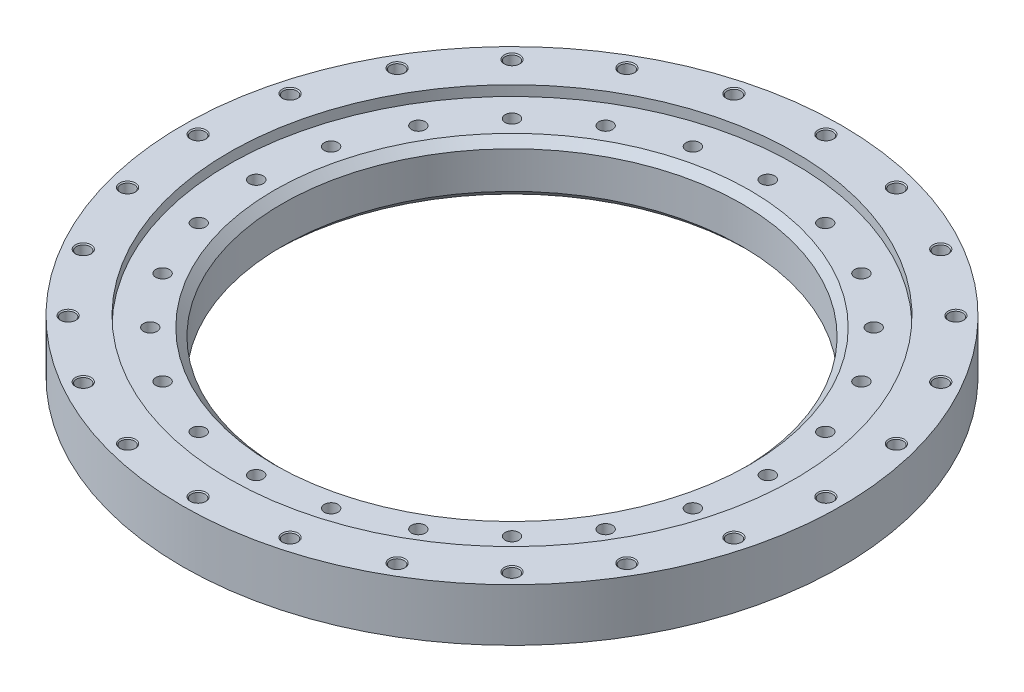
SolidWorks part; units mm, degrees
ref_plane "Front Plane" through (0, 0, 0) normal (0, 0, 1) x (1, 0, 0)
ref_plane "Top Plane" through (0, 0, 0) normal (0, 1, 0) x (1, 0, 0)
ref_plane "Right Plane" through (0, 0, 0) normal (1, 0, 0) x (0, 0, -1)
sketch "Sketch1" plane through (0, 0, 0) normal (0, 1, 0) x (1, 0, 0)
  circle A0 centre (0, 0) radius 420
  dimension "D1" = 840
extrude "Boss-Extrude1" add sketch "Sketch1" along normal blind 67
sketch "Sketch2" plane through (0, 67, 0) normal (0, 1, 0) x (1, 0, 0)
  circle A0 centre (0, 0) radius 360.5
  dimension "D1" = 721
extrude "Cut-Extrude1" cut sketch "Sketch2" against normal blind 13
sketch "Sketch3" plane through (0, 0, 0) normal (0, -1, 0) x (1, 0, 0)
  circle A0 centre (0, 0) radius 360
  dimension "D1" = 720
extrude "Boss-Extrude2" add sketch "Sketch3" along normal blind 13
hole_wizard "M20 Tapped Hole1" positions "Sketch4" profile "Sketch5" tap size "M20" standard "GB" end condition through all
sketch "Sketch4" plane through (0, 67, 0) normal (0, 1, 0) x (1, 0, 0)
  circle A0 centre (0, 0) radius 400 construction
  point P8 (0, 400)
  point P14 (103.5276, 386.3703)
  point P15 (200, 346.4102)
  point P16 (282.8427, 282.8427)
  point P17 (346.4102, 200)
  point P18 (386.3703, 103.5276)
  point P19 (400, 0)
  point P20 (386.3703, -103.5276)
  point P21 (346.4102, -200)
  point P22 (282.8427, -282.8427)
  point P23 (200, -346.4102)
  point P24 (103.5276, -386.3703)
  point P25 (0, -400)
  point P26 (-103.5276, -386.3703)
  point P27 (-200, -346.4102)
  point P28 (-282.8427, -282.8427)
  point P29 (-346.4102, -200)
  point P30 (-386.3703, -103.5276)
  point P31 (-400, 0)
  point P32 (-386.3703, 103.5276)
  point P33 (-346.4102, 200)
  point P34 (-282.8427, 282.8427)
  point P35 (-200, 346.4102)
  point P36 (-103.5276, 386.3703)
  dimension "D2" = 24
sketch "Sketch5" plane through (-103.5276, 67, -386.3703) normal (1, 0, 0) x (0, 0, 1)
  line L0 (0, 0) -> (0, 80)
  line L1 (0, 80) -> (8.75, 80)
  line L2 (8.75, 80) -> (8.75, 1.275)
  line L3 (8.75, 1.275) -> (10.025, 0)
  line L5 (10.025, 0) -> (0, 0)
  line L6 (-8.75, 1.275) -> (-10.025, 0) construction
  line L11 (0, -6.35) -> (0, 107.95) construction
  dimension "通孔螺纹孔钻头直径" = 17.5
  dimension "通孔螺纹孔钻头深度" = 80
  dimension "近端锥形沉头孔直径" = 20.05
  dimension "近端锥形沉头孔角度" = 90
cosmetic thread "Cosmetic thread 1" parameters "D2"=20
cosmetic thread "Cosmetic thread 2" parameters "D2"=20
cosmetic thread "Cosmetic thread 3" parameters "D2"=20
cosmetic thread "Cosmetic thread 4" parameters "D2"=20
cosmetic thread "Cosmetic thread 5" parameters "D2"=20
cosmetic thread "Cosmetic thread 6" parameters "D2"=20
cosmetic thread "Cosmetic thread 7" parameters "D2"=20
cosmetic thread "Cosmetic thread 8" parameters "D2"=20
cosmetic thread "Cosmetic thread 9" parameters "D2"=20
cosmetic thread "Cosmetic thread 10" parameters "D2"=20
cosmetic thread "Cosmetic thread 11" parameters "D2"=20
cosmetic thread "Cosmetic thread 12" parameters "D2"=20
cosmetic thread "Cosmetic thread 13" parameters "D2"=20
cosmetic thread "Cosmetic thread 14" parameters "D2"=20
cosmetic thread "Cosmetic thread 15" parameters "D2"=20
cosmetic thread "Cosmetic thread 16" parameters "D2"=20
cosmetic thread "Cosmetic thread 17" parameters "D2"=20
cosmetic thread "Cosmetic thread 18" parameters "D2"=20
cosmetic thread "Cosmetic thread 19" parameters "D2"=20
cosmetic thread "Cosmetic thread 20" parameters "D2"=20
cosmetic thread "Cosmetic thread 21" parameters "D2"=20
cosmetic thread "Cosmetic thread 22" parameters "D2"=20
cosmetic thread "Cosmetic thread 23" parameters "D2"=20
cosmetic thread "Cosmetic thread 24" parameters "D2"=20
sketch "Sketch6" plane through (0, 54, 0) normal (0, 1, 0) x (1, 0, 0)
  circle A0 centre (0, 0) radius 293
  dimension "D1" = 586
extrude "Cut-Extrude2" cut sketch "Sketch6" against normal through all
chamfer "Chamfer1" distance 10 angle 45 2 edges at (0, -13, 293) (0, 54, 293)
hole_wizard "M20 Tapped Hole2" positions "Sketch7" profile "Sketch8" tap size "M20" standard "GB" end condition through all
sketch "Sketch7" plane through (0, -13, 0) normal (0, -1, 0) x (-1, 0, 0)
  circle A0 centre (0, 0) radius 326 construction
  point P5 (0, 326)
  point P12 (84.375, 314.8918)
  point P13 (163, 282.3243)
  point P14 (230.5168, 230.5168)
  point P15 (282.3243, 163)
  point P16 (314.8918, 84.375)
  point P17 (326, 0)
  point P18 (314.8918, -84.375)
  point P19 (282.3243, -163)
  point P20 (230.5168, -230.5168)
  point P21 (163, -282.3243)
  point P22 (84.375, -314.8918)
  point P23 (0, -326)
  point P24 (-84.375, -314.8918)
  point P25 (-163, -282.3243)
  point P26 (-230.5168, -230.5168)
  point P27 (-282.3243, -163)
  point P28 (-314.8918, -84.375)
  point P29 (-326, 0)
  point P30 (-314.8918, 84.375)
  point P31 (-282.3243, 163)
  point P32 (-230.5168, 230.5168)
  point P33 (-163, 282.3243)
  point P34 (-84.375, 314.8918)
  dimension "D2" = 24
sketch "Sketch8" plane through (84.375, -13, -314.8918) normal (1, 0, 0) x (0, 0, -1)
  line L0 (0, 0) -> (0, 80)
  line L1 (0, 80) -> (8.75, 80)
  line L2 (8.75, 80) -> (8.75, 1.275)
  line L3 (8.75, 1.275) -> (10.025, 0)
  line L5 (10.025, 0) -> (0, 0)
  line L6 (-8.75, 1.275) -> (-10.025, 0) construction
  line L11 (0, -6.35) -> (0, 107.95) construction
  dimension "通孔螺纹孔钻头直径" = 17.5
  dimension "通孔螺纹孔钻头深度" = 80
  dimension "近端锥形沉头孔直径" = 20.05
  dimension "近端锥形沉头孔角度" = 90
cosmetic thread "Cosmetic thread 25" parameters "D2"=20
cosmetic thread "Cosmetic thread 26" parameters "D2"=20
cosmetic thread "Cosmetic thread 27" parameters "D2"=20
cosmetic thread "Cosmetic thread 28" parameters "D2"=20
cosmetic thread "Cosmetic thread 29" parameters "D2"=20
cosmetic thread "Cosmetic thread 30" parameters "D2"=20
cosmetic thread "Cosmetic thread 31" parameters "D2"=20
cosmetic thread "Cosmetic thread 32" parameters "D2"=20
cosmetic thread "Cosmetic thread 33" parameters "D2"=20
cosmetic thread "Cosmetic thread 34" parameters "D2"=20
cosmetic thread "Cosmetic thread 35" parameters "D2"=20
cosmetic thread "Cosmetic thread 36" parameters "D2"=20
cosmetic thread "Cosmetic thread 37" parameters "D2"=20
cosmetic thread "Cosmetic thread 38" parameters "D2"=20
cosmetic thread "Cosmetic thread 39" parameters "D2"=20
cosmetic thread "Cosmetic thread 40" parameters "D2"=20
cosmetic thread "Cosmetic thread 41" parameters "D2"=20
cosmetic thread "Cosmetic thread 42" parameters "D2"=20
cosmetic thread "Cosmetic thread 43" parameters "D2"=20
cosmetic thread "Cosmetic thread 44" parameters "D2"=20
cosmetic thread "Cosmetic thread 45" parameters "D2"=20
cosmetic thread "Cosmetic thread 46" parameters "D2"=20
cosmetic thread "Cosmetic thread 47" parameters "D2"=20
cosmetic thread "Cosmetic thread 48" parameters "D2"=20
